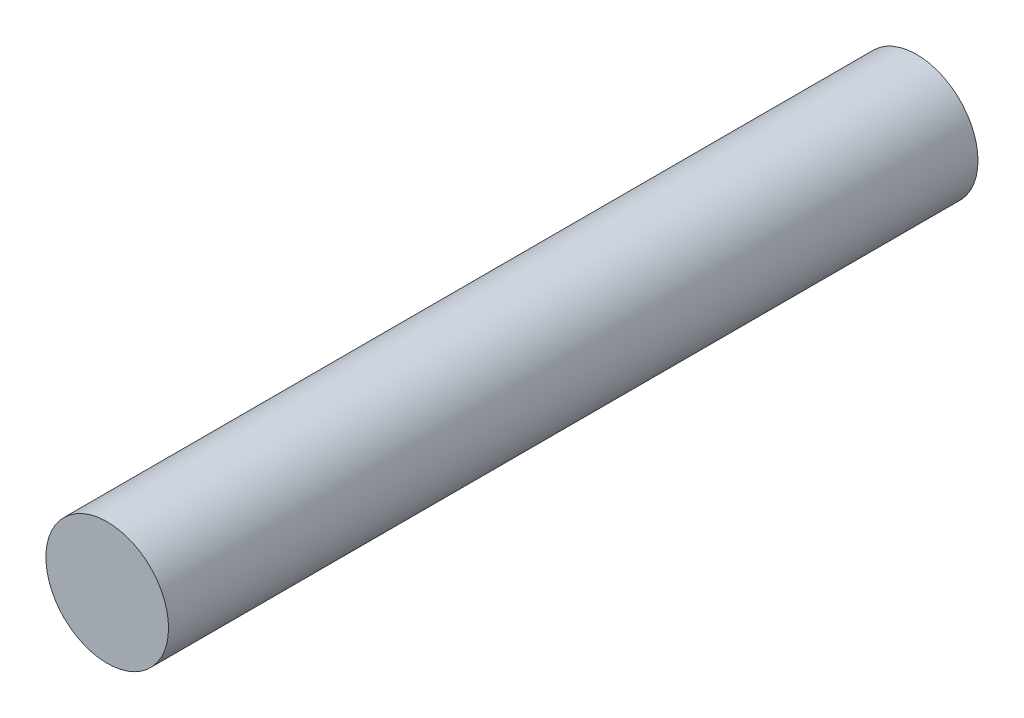
from build123d import *

# Parameters (mm, degrees)
SKETCH_1_R      = 12.5
EXTRUDE_1_DEPTH = 165


with BuildPart() as part:
    # 草图1 → 凸台-拉伸1 (new body)
    with BuildSketch(Plane.XY):
        Circle(SKETCH_1_R)
    extrude(amount=EXTRUDE_1_DEPTH)


solid = part.part
